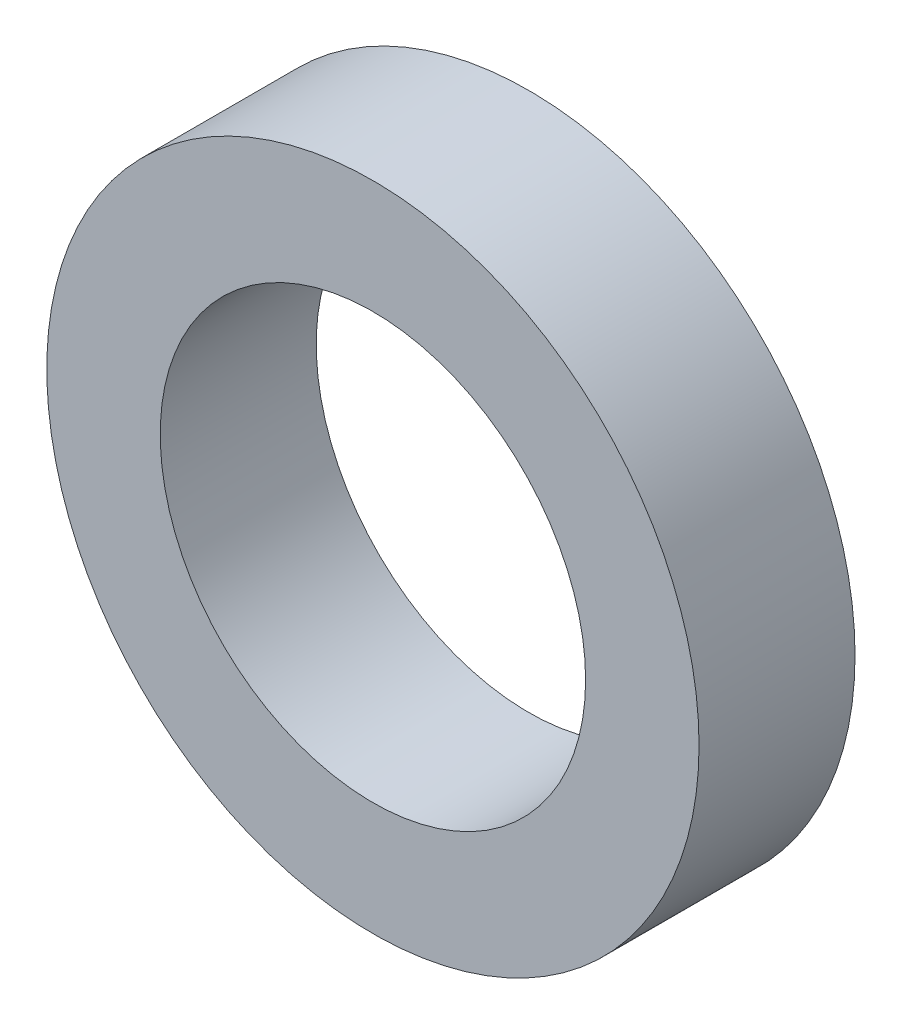
SolidWorks part; units mm, degrees
ref_plane "Front Plane" through (0, 0, 0) normal (0, 0, 1) x (1, 0, 0)
ref_plane "Top Plane" through (0, 0, 0) normal (0, 1, 0) x (1, 0, 0)
ref_plane "Right Plane" through (0, 0, 0) normal (1, 0, 0) x (0, 0, -1)
sketch "Sketch1" plane through (0, 0, 0) normal (0, 0, 1) x (1, 0, 0)
  circle A0 centre (0, 0) radius 46
  circle A1 centre (0, 0) radius 30
  dimension "D1" = 92
  dimension "D2" = 60
extrude "Boss-Extrude1" add sketch "Sketch1" along normal blind 22
